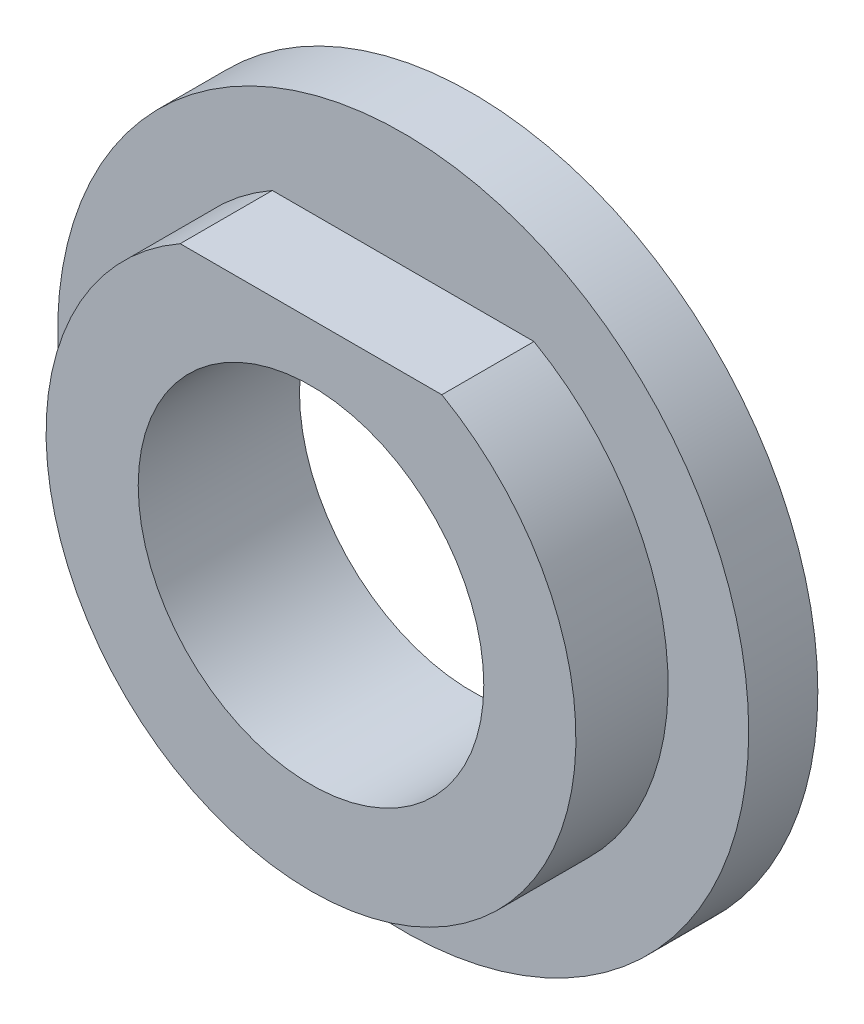
SolidWorks part; units mm, degrees
ref_plane "前视基准面" through (0, 0, 0) normal (0, 0, 1) x (1, 0, 0)
ref_plane "上视基准面" through (0, 0, 0) normal (0, 1, 0) x (1, 0, 0)
ref_plane "右视基准面" through (0, 0, 0) normal (1, 0, 0) x (0, 0, -1)
sketch "草图1" plane through (0, 0, 0) normal (0, 0, 1) x (1, 0, 0)
  circle A0 centre (0, 0) radius 15
  circle A1 centre (0, 0) radius 7.5
  dimension "D1" = 30
  dimension "D2" = 15
extrude "凸台-拉伸1" add sketch "草图1" along normal blind 7
sketch "草图2" plane through (0, 0, 7) normal (0, 0, 1) x (1, 0, 0)
  line L0 (0, -11.5) -> (0, 10) construction
  line L1 (-5.6789, 10) -> (5.6789, 10)
  circle A0 centre (0, 0) radius 15
  arc A1 (-5.6789, 10) -> (5.6789, 10) centre (0, 0) ccw
  point P9 (0, 10)
  dimension "D1" = 23
  dimension "D2" = 21.5
extrude "切除-拉伸2" cut sketch "草图2" against normal blind 4
